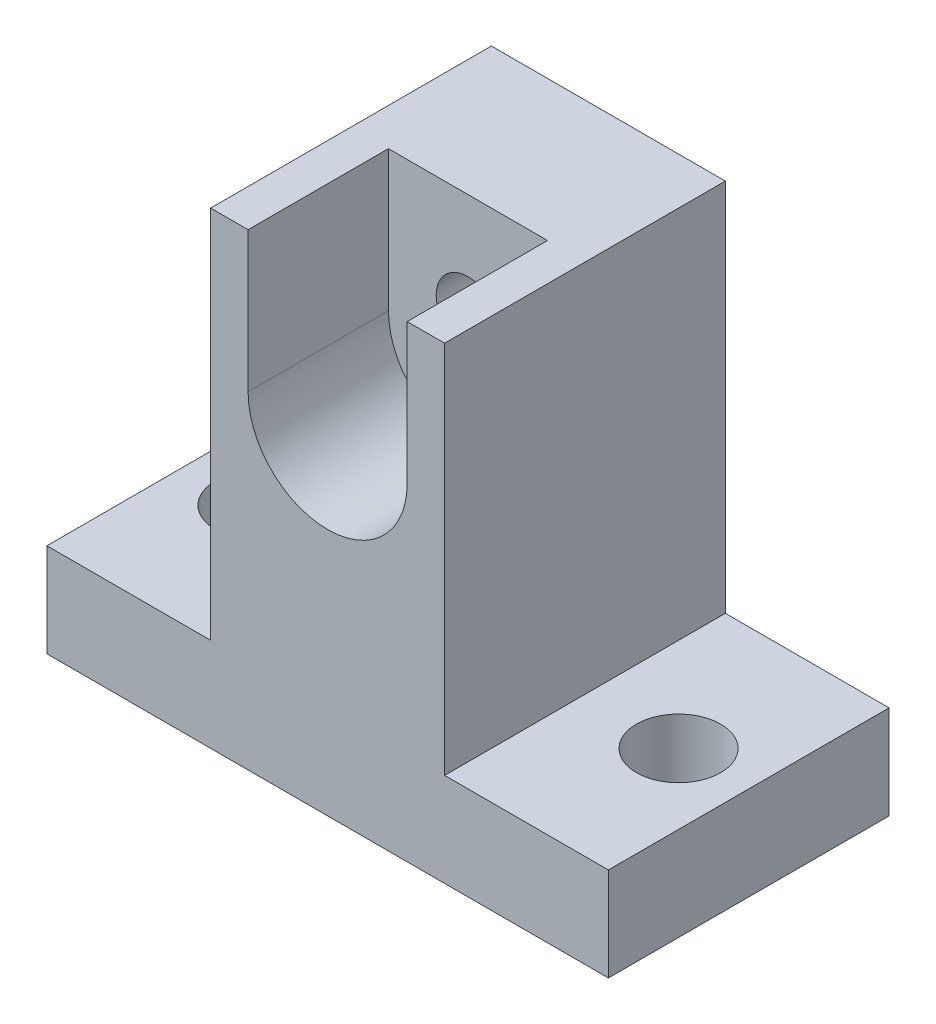
from build123d import *

# Parameters (mm, degrees)
BOSS_EXTRUDE1_DEPTH          = 30
CUT_EXTRUDE1_DEPTH           = 15
F_9_0_9_DIAMETER_HOLE1_D     = 9
F_9_0_9_DIAMETER_HOLE1_DEPTH = 10
F_9_0_9_DIAMETER_HOLE1_TIP   = 2.703872786
M8_TAPPED_HOLE1_D            = 6.8


with BuildPart() as part:
    # Sketch1 → Boss-Extrude1 (new body)
    with BuildSketch(Plane.XY):
        Polygon((0, 0), (0, 10), (17.5, 10), (17.5, 50), (42.5, 50), (42.5, 10), (60, 10), (60, 0), align=None)
    extrude(amount=BOSS_EXTRUDE1_DEPTH)

    # Sketch2 → Cut-Extrude1 (cut)
    with BuildSketch(Plane.XY.offset(30)):
        with BuildLine():
            Line((38.5, 50), (38.5, 35))
            ThreePointArc((38.5, 35), (30, 26.5), (21.5, 35))
            Line((21.5, 35), (21.5, 50))
            ThreePointArc((21.5, 50), (30, 58.5), (38.5, 50))
        make_face()
    extrude(amount=-CUT_EXTRUDE1_DEPTH, mode=Mode.SUBTRACT)

    # Ø9.0 (9) Diameter Hole1
    with Locations(Plane(origin=(7.5, 0, 15), x_dir=(-1, 0, 0), z_dir=(0, -1, 0))):
        with Locations((0, 0), (-45, 0)):
            Hole(F_9_0_9_DIAMETER_HOLE1_D / 2, depth=F_9_0_9_DIAMETER_HOLE1_DEPTH)
            with Locations((0, 0, -(F_9_0_9_DIAMETER_HOLE1_DEPTH + F_9_0_9_DIAMETER_HOLE1_TIP / 2))):  # 118° drill point
                Cone(0, F_9_0_9_DIAMETER_HOLE1_D / 2, F_9_0_9_DIAMETER_HOLE1_TIP, mode=Mode.SUBTRACT)

    # M8 Tapped Hole1 (through all)
    with Locations(Plane(origin=(30, 39, 0), x_dir=(-1, 0, 0), z_dir=(0, 0, -1))):
        with Locations((0, 0)):
            Hole(M8_TAPPED_HOLE1_D / 2)


solid = part.part
